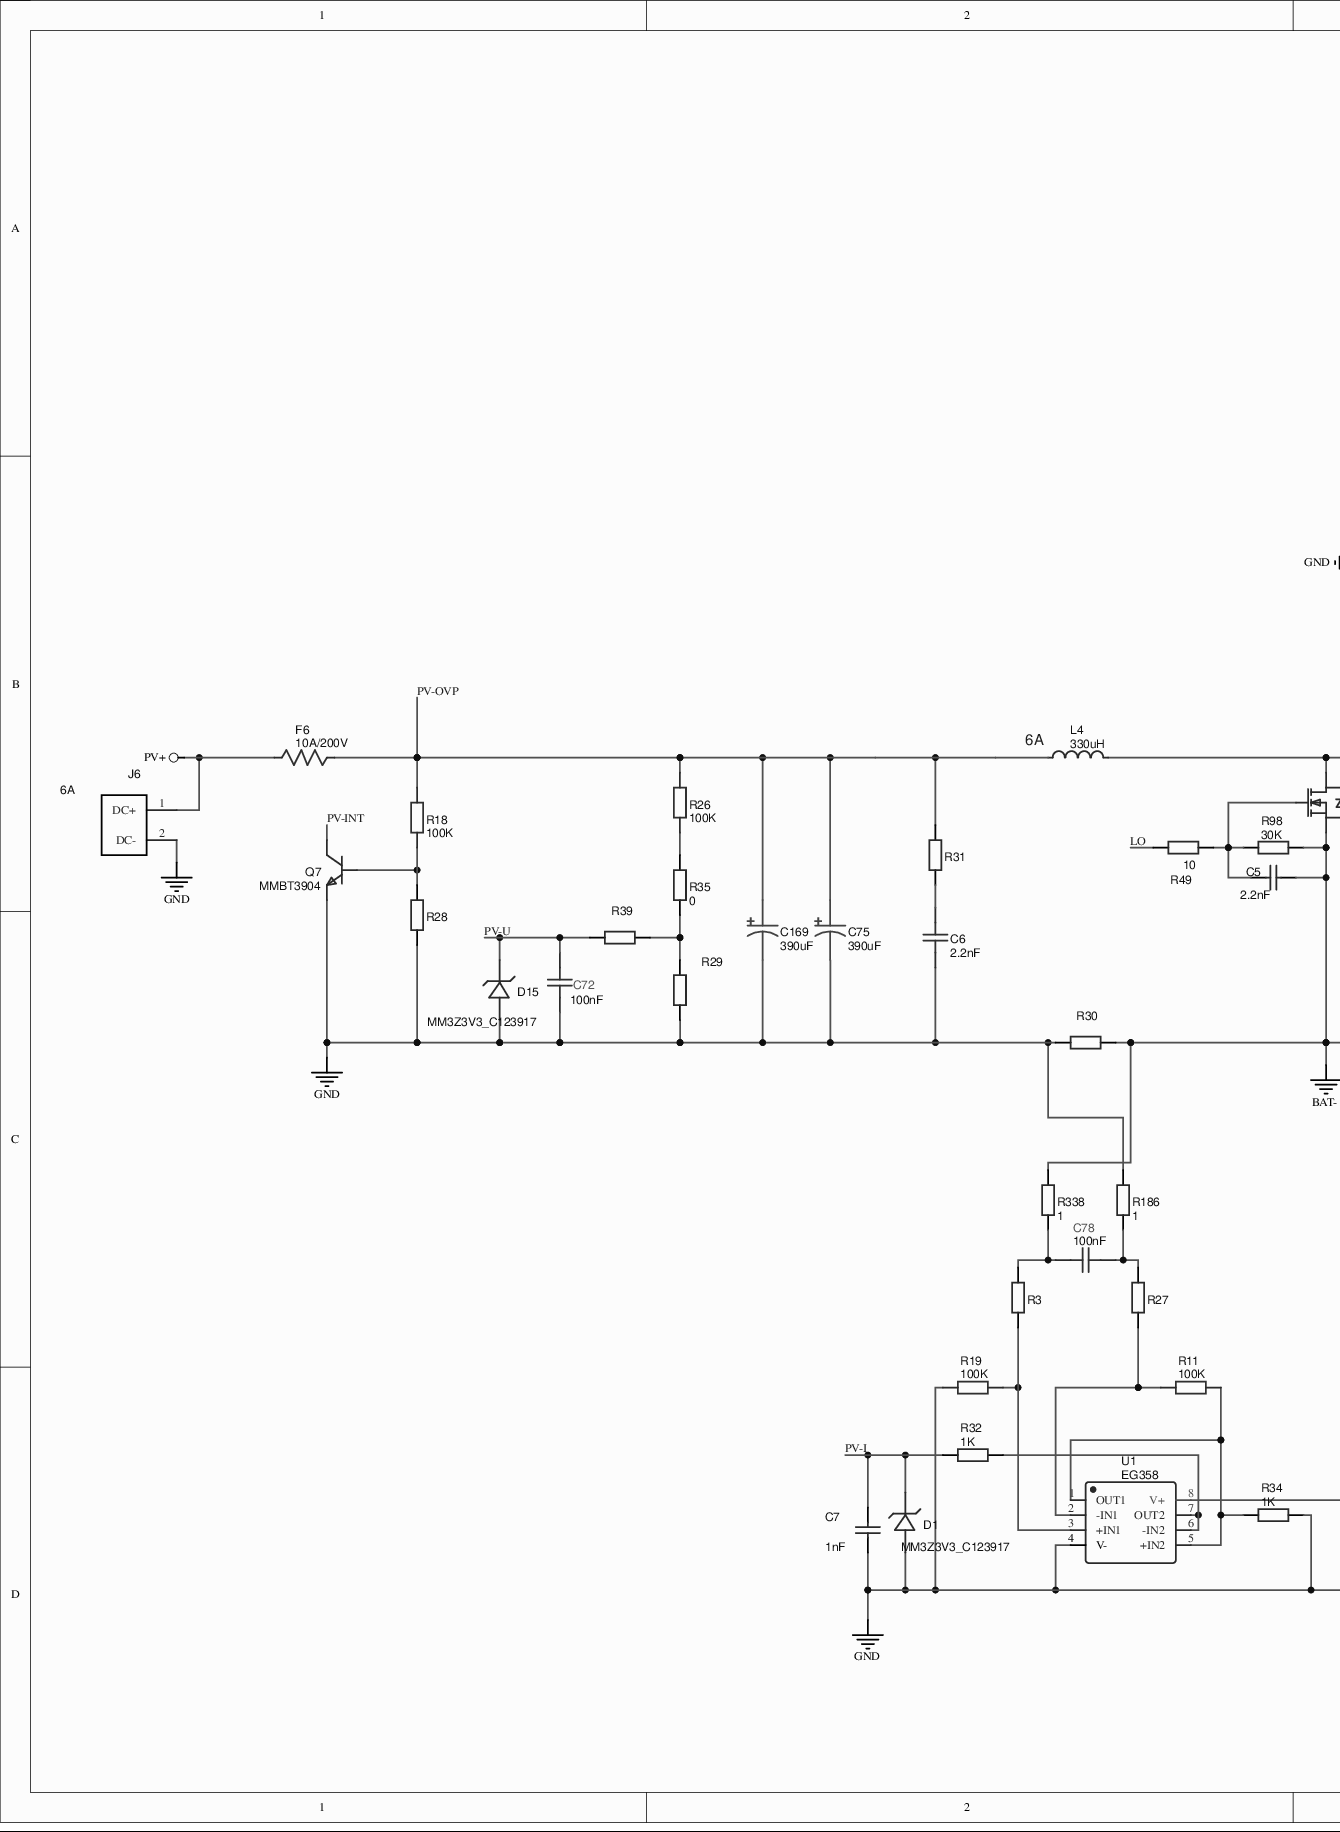
[diagram p0: MISC84449-3.SchDoc, left]
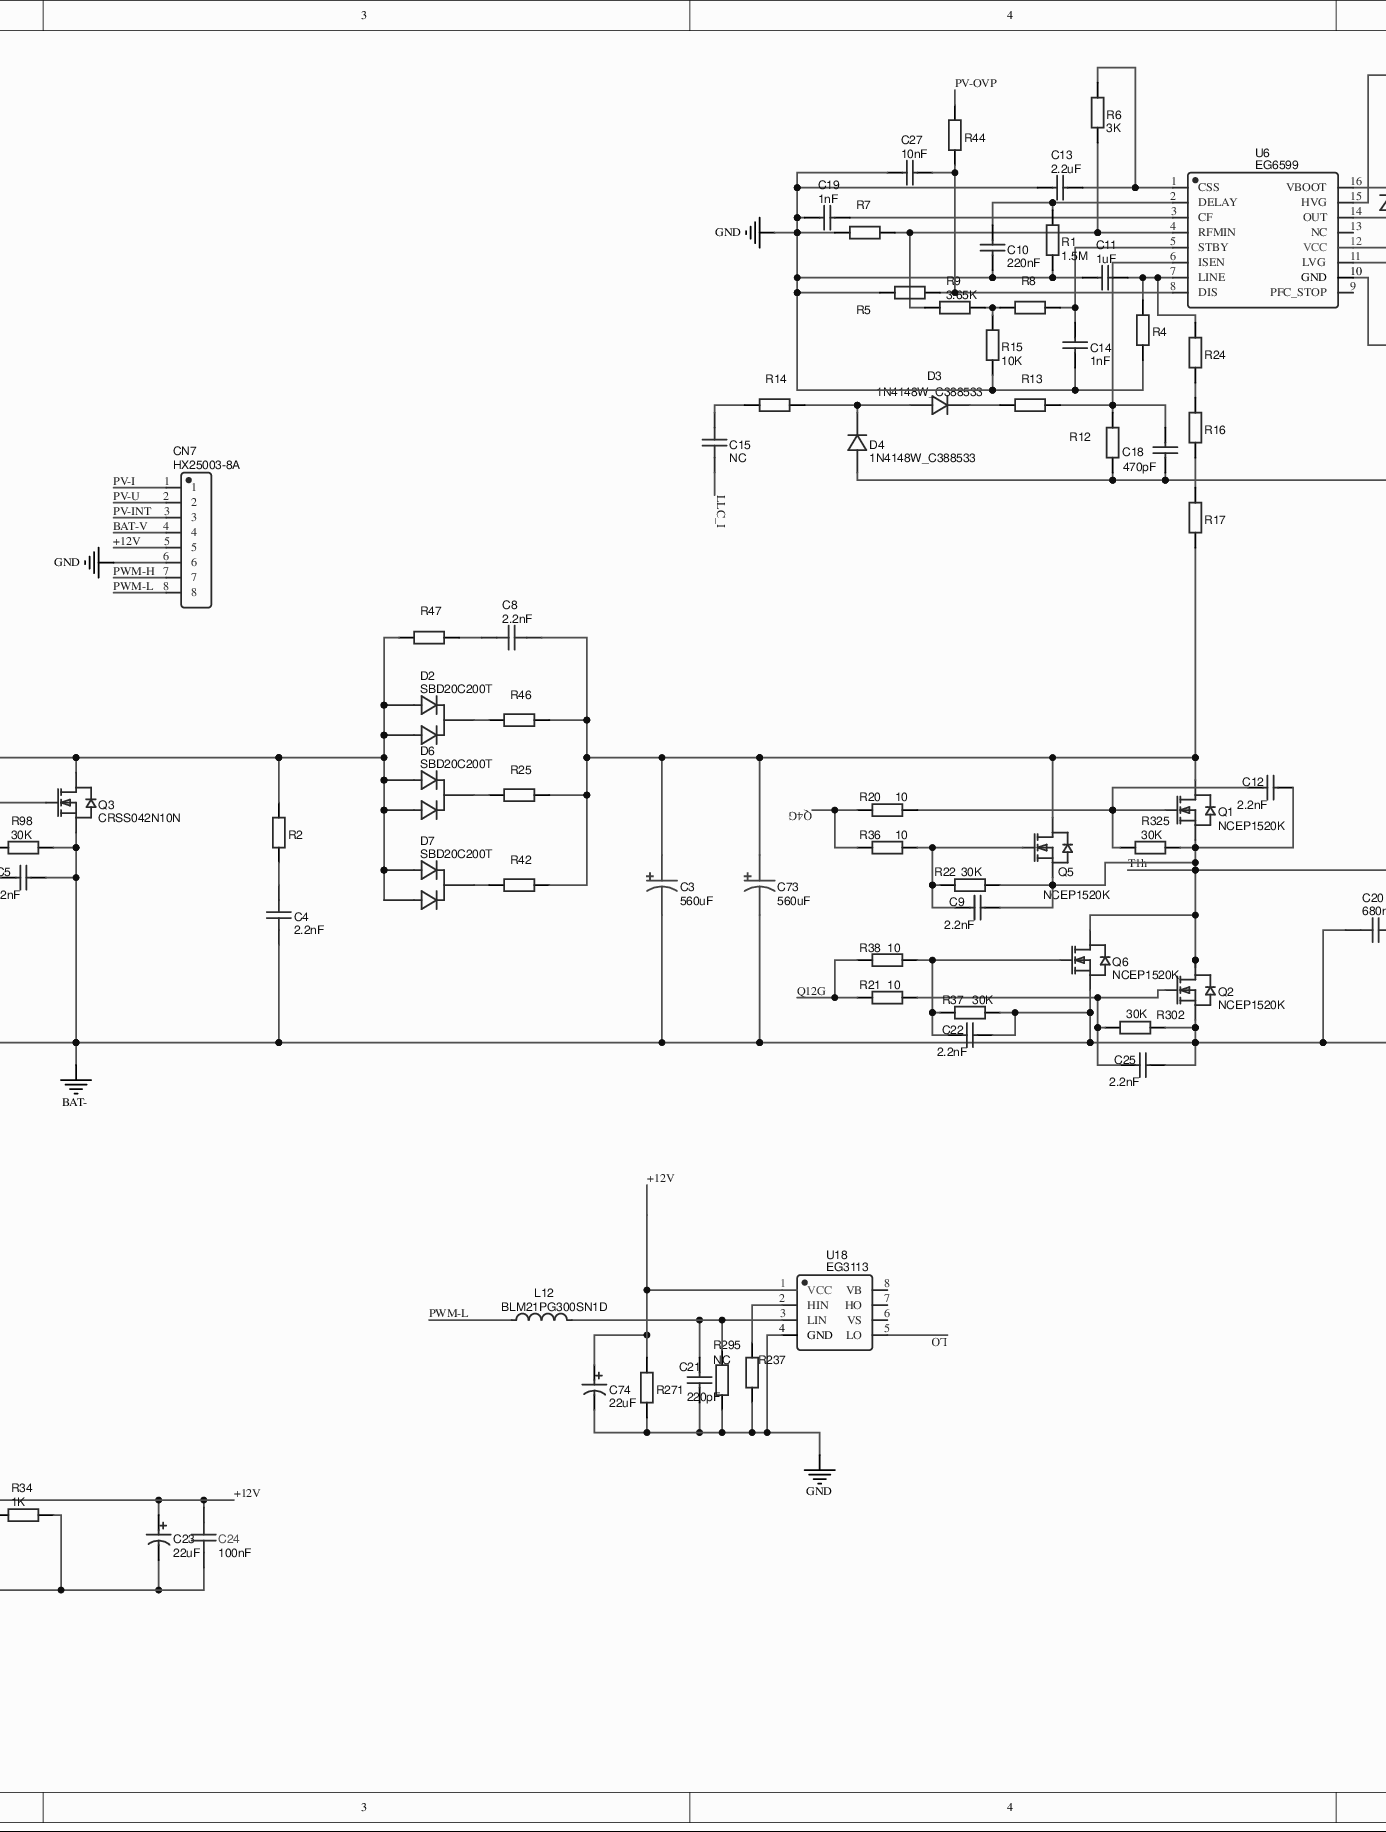
[diagram p1: MISC84449-3.SchDoc, middle]
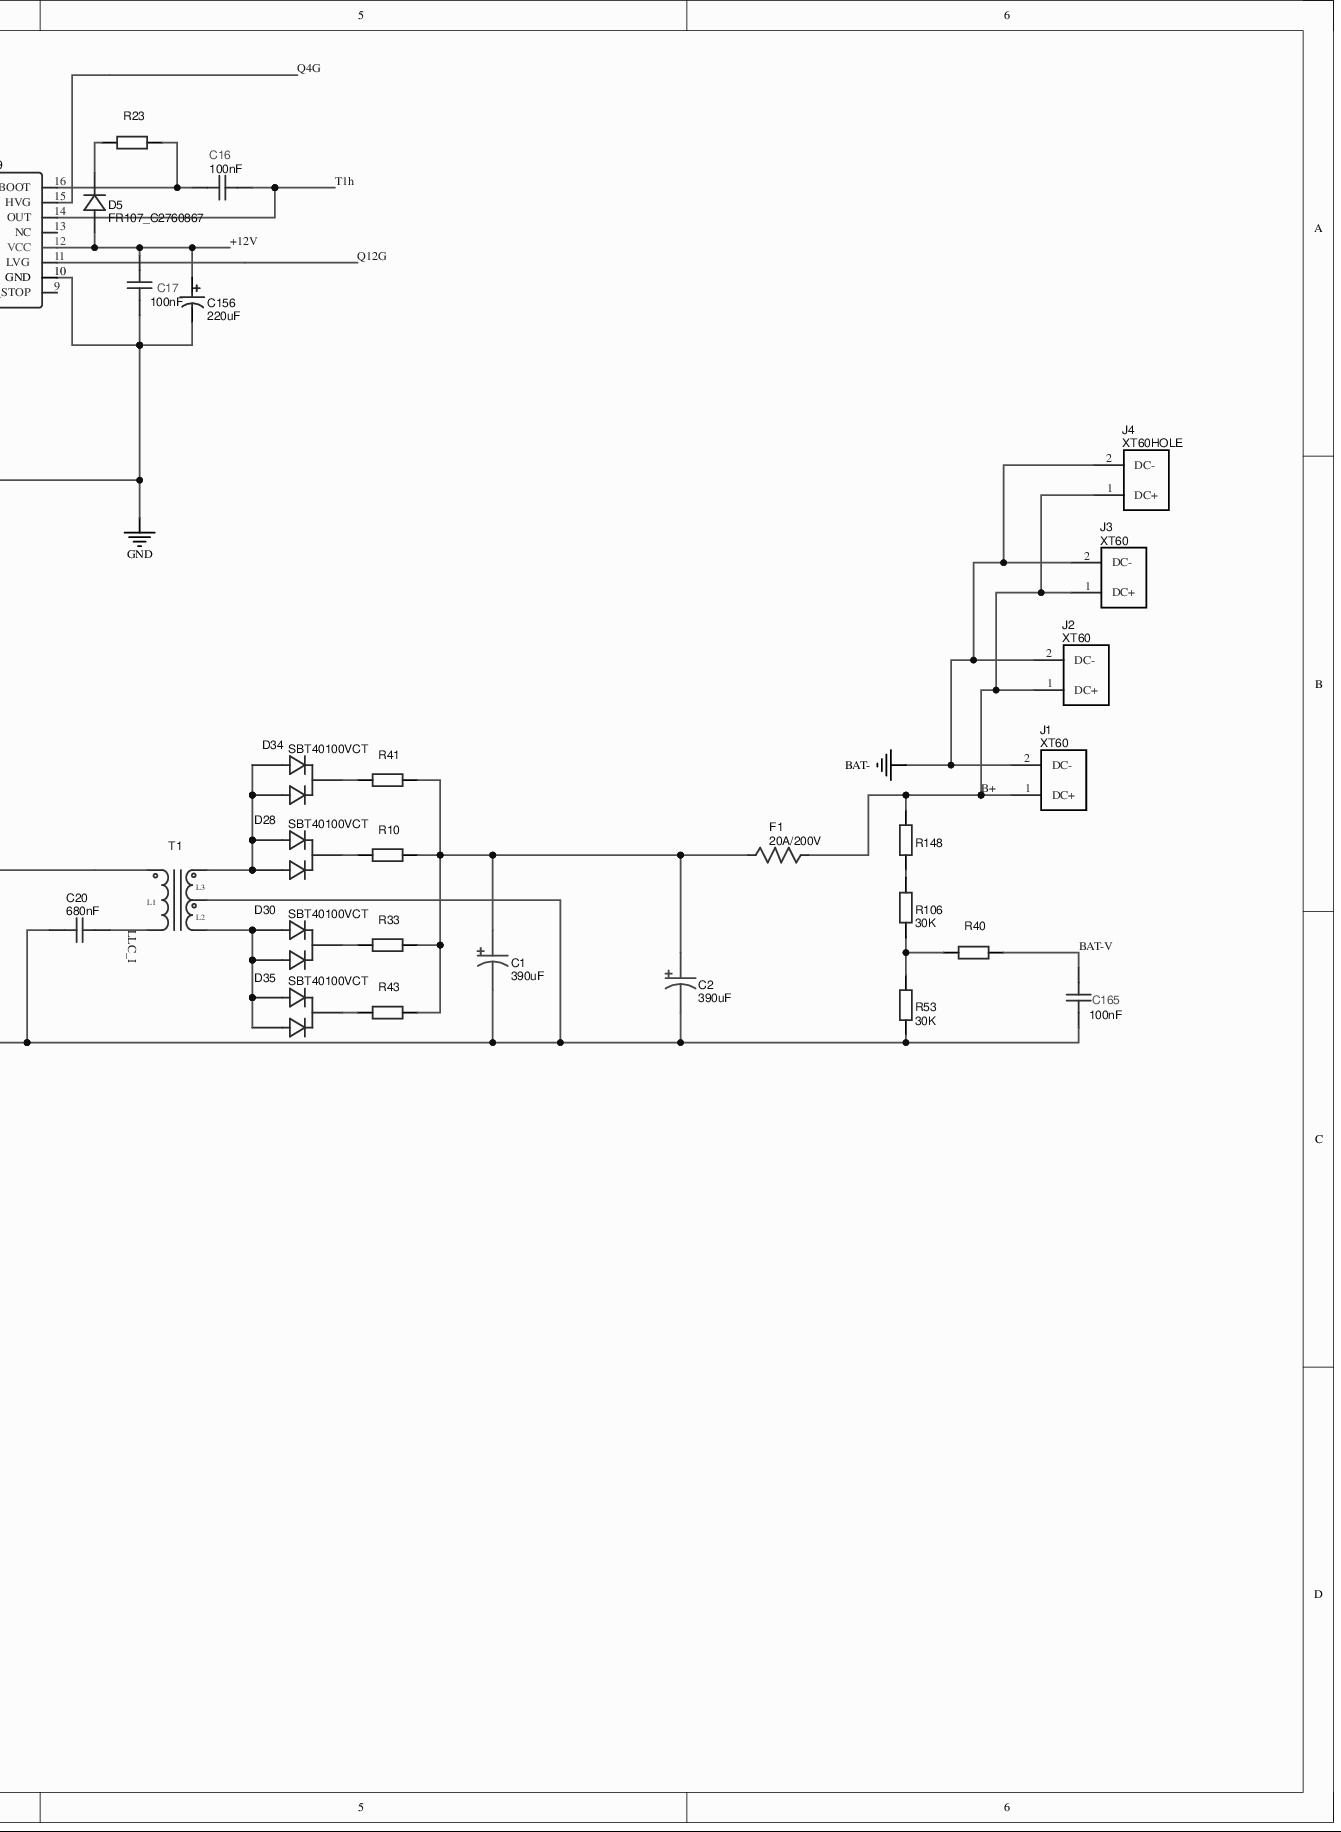
[diagram p2: MISC84449-3.SchDoc, right]
# Altium project MISC84449-4.PrjPcb
1 sheet, 124 parts. Net scope: global (net labels, ports and power ports of the same name join across sheets).
Board file: MISC84449.PcbDoc

## Sheet MISC84449-3.SchDoc
size 655 x 308 mm

### Parts
C1  390uF  [CAP-TH_BD8.0-P3.50-D0.6-FD]
C2  390uF  [CAP-TH_BD8.0-P3.50-D0.6-FD]
C3  560uF  [CAP-TH_BD12.5-P5.00-D0.6-FD]
C4  2.2nF  [C1206]
C5  2.2nF  [C0603]
C6  2.2nF  [C1206]
C7  1nF  [C0603]
C8  2.2nF  [C1206]
C9  2.2nF  [C0603]
C10  220nF  [C0603]
C11  1uF  [C0603]
C12  2.2nF  [C0603]
C13  2.2uF  [C0603]
C14  1nF  [C0603]
C15  NC  [C1206]
C16  100nF  [C0603]
C17  100nF  [C0603]
C18  470pF  [C0603]
C19  1nF  [C0603]
C20  680nF  [CAP-TH_L17.5-W8.5-P15.00-D0.8]
C21  220pF  [C0603]
C22  2.2nF  [C0603]
C23  22uF  [CAP-TH_BD5.0-P2.00-D0.8-FD]
C24  100nF  [C0603]
C25  2.2nF  [C0603]
C27  10nF  [C1206]
C72  100nF  [C0603]
C73  560uF  [CAP-TH_BD12.5-P5.00-D0.6-FD]
C74  22uF  [CAP-TH_BD5.0-P2.00-D0.8-FD]
C75  390uF  [CAP-TH_BD10.0-P5.00-D1.0-FD]
C78  100nF  [C0603]
C156  220uF  [CAP-TH_BD6.3-P2.50-D1.0-FD]
C165  100nF  [C0603]
C169  390uF  [CAP-TH_BD10.0-P5.00-D1.0-FD]
CN7  HX25003-8A  [CONN-TH_8P-P2.50_HX25003-8A]
D1  MM3Z3V3_C123917  [SOD-323_L1.8-W1.3-LS2.5-RD]
D2  SBD20C200T  [TO-220-3_L10.0-W4.5-P2.54-L]
D3  1N4148W_C388533  [SOD-123_L2.8-W1.8-LS3.7-RD]
D4  1N4148W_C388533  [SOD-123_L2.8-W1.8-LS3.7-RD]
D5  FR107_C2760867  [SOD-123FL_L2.7-W1.8-LS3.8-RD]
D6  SBD20C200T  [TO-220-3_L10.0-W4.5-P2.54-L]
D7  SBD20C200T  [TO-220-3_L10.0-W4.5-P2.54-L]
D15  MM3Z3V3_C123917  [SOD-323_L1.8-W1.3-LS2.5-RD]
D28  SBT40100VCT  [TO-220-3_L10.0-W4.5-P2.54-L]
D30  SBT40100VCT  [TO-220-3_L10.0-W4.5-P2.54-L]
D34  SBT40100VCT  [TO-220-3_L10.0-W4.5-P2.54-L]
D35  SBT40100VCT  [TO-220-3_L10.0-W4.5-P2.54-L]
F1  20A/200V  [FUSE-SMD_L6.1-W2.5]
F6  10A/200V  [FUSE-SMD_L6.1-W2.5]
J1  XT60  [CONN-TH_XT60UPB-F]
J2  XT60  [CONN-TH_XT60UPB-F]
J3  XT60  [CONN-TH_XT60UPB-F]
J4  XT60HOLE  [XT90N]
J6  6A  [CONN-TH_XT60UPB-F]
L4  330uH  [200W-TMS330060A]
L12  BLM21PG300SN1D  [L0805]
Q1  NCEP1520K  [TO-252-2_L6.6-W6.1-P4.57-LS9.9-BR-CW]
Q2  NCEP1520K  [TO-252-2_L6.6-W6.1-P4.57-LS9.9-BR-CW]
Q3  CRSS042N10N  [TO-263-3_L10.2-W10.7-P5.08-LS16.2-TL]
Q5  NCEP1520K  [TO-252-2_L6.6-W6.1-P4.57-LS9.9-BR-CW]
Q6  NCEP1520K  [TO-252-2_L6.6-W6.1-P4.57-LS9.9-BR-CW]
Q7  MMBT3904  [SOT-23-3_L2.9-W1.3-P1.90-LS2.4-BR]
R1  1.5M  [R0603]
R2  (no value)  [R1206]
R3  (no value)  [R0603]
R4  (no value)  [R0603]
R5  (no value)  [R0805]
R6  3K  [R0603]
R7  (no value)  [R0603]
R8  (no value)  [R0603]
R9  3.65K  [R0603]
R10  (no value)  [R2512]
R11  100K  [R0805]
R12  (no value)  [R0603]
R13  (no value)  [R0603]
R14  (no value)  [R0603]
R15  10K  [R1206]
R16  (no value)  [R0603]
R17  (no value)  [R1206]
R18  100K  [R0805]
R19  100K  [R0805]
R20  10  [R1206]
R21  10  [R1206]
R22  30K  [R0603]
R23  (no value)  [R0805]
R24  (no value)  [R0603]
R25  (no value)  [R2512]
R26  100K  [R0805]
R27  (no value)  [R0603]
R28  (no value)  [R0805]
R29  (no value)  [R0603]
R30  (no value)  [R2512]
R31  (no value)  [R1206]
R32  1K  [R0603]
R33  (no value)  [R2512]
R34  1K  [R0603]
R35  0  [R0805]
R36  10  [R1206]
R37  30K  [R0603]
R38  10  [R1206]
R39  (no value)  [R0805]
R40  (no value)  [R0805]
R41  (no value)  [R2512]
R42  (no value)  [R2512]
R43  (no value)  [R2512]
R44  (no value)  [R0805]
R46  (no value)  [R2512]
R47  (no value)  [R1206]
R49  10  [R0603]
R53  30K  [R0603]
R98  30K  [R0603]
R106  30K  [R0603]
R148  (no value)  [R0603]
R186  1  [R0603]
R237  (no value)  [R0603]
R271  (no value)  [R0603]
R295  NC  [R0603]
R302  30K  [R0603]
R325  30K  [R0603]
R338  1  [R0603]
T1  (no value)  [PQ3230 3:2:2-N]
U1  EG358  [SOIC-8_L5.0-W4.0-P1.27-LS6.0-BL]
U6  EG6599  [SO-16_L10.0-W4.0-P1.27-LS6.2-BL]
U18  EG3113  [SOP-8_L4.9-W3.9-P1.27-LS6.0-BL]

### Nets
BAT-: C1.2 C2.2 C3.2 C4.2 C5.2 C20.2 C22.2 C25.2 C73.2 C165.1 J1.2(DC-) J2.2(DC-) J3.2(DC-) J4.2(DC-) Q2.3(S) Q3.3(S) Q6.3(S) R30.2 R37.2 R53.1 R98.1 R302.2 R338.2 T1.9
GND: C6.2 C7.1 C10.1 C11.2 C13.1 C14.1 C17.1 C18.1 C19.2 C21.1 C23.2 C24.2 C27.1 C72.1 C74.2 C75.2 C156.2 C169.2 CN7.6 D1.2(A) D4.2(A) D15.2(A) J6.2(DC-) Q7.2(E) R1.1 R4.1 R5.1 R7.2 R12.1 R15.2 R19.2 R28.1 R29.1 R30.1 R34.2 R186.2 R237.1 R271.1 R295.2 U1.4(V-) U6.10(GND) U18.4(GND)
PV+: F6.1 J6.1(DC+)
+12V: C17.2 C23.1 C24.1 C74.1 C156.1 CN7.5 D5.2(A) R271.2 U1.8(V+) U6.12(VCC) U18.1(VCC)
B+: F1.2 J1.1(DC+) J2.1(DC+) J3.1(DC+) J4.1(DC+) R148.2
BAT-V: C165.2 CN7.4 R40.2
LLC_I: C15.1 C20.1 T1.3
LO: R49.2 U18.5(LO)
PV-I: C7.2 CN7.1 D1.1(K) R32.2
PV-INT: CN7.3 Q7.3(C)
PV-OVP: C75.1 C169.1 F6.2 L4.1 R18.2 R26.2 R31.1 R44.2
PV-U: C72.2 CN7.2 D15.1(K) R39.1
PWM-H: CN7.7
PWM-L: CN7.8 L12.1
Q4G: R20.1 R36.1 U6.15(HVG)
Q12G: R21.1 R38.1 U6.11(LVG)
T1h: C9.2 C12.2 C16.1 Q1.3(S) Q2.2(D) Q5.3(S) Q6.2(D) R22.2 R325.2 T1.4 U6.14(OUT)
NetC1_1: C1.1 C2.1 F1.1 R10.2 R33.2 R41.2 R43.2
NetC3_1: C3.1 C8.2 C73.1 Q1.2(D) Q5.2(D) R17.1 R25.2 R42.2 R46.2
NetC4_1: C4.1 R2.2
NetC5_1: C5.1 Q3.1(G) R49.1 R98.2
NetC6_1: C6.1 R31.2
NetC8_1: C8.1 R47.2
NetC9_1: C9.1 Q5.1(G) R22.1 R36.2
NetC10_2: C10.2 R1.2 U6.2(DELAY)
NetC11_1: C11.1 R4.2 R24.2 U6.7(LINE)
NetC12_1: C12.1 Q1.1(G) R20.2 R325.1
NetC13_2: C13.2 R6.2 U6.1(CSS)
NetC14_2: C14.2 R8.2 U6.5(STBY)
NetC15_2: C15.2 R14.1
NetC16_2: C16.2 R23.1 U6.16(VBOOT)
NetC18_2: C18.2 R12.2 R13.2 U6.6(ISEN)
NetC19_1: C19.1 U6.3(CF)
NetC21_2: C21.2 L12.2 R295.1 U18.3(LIN)
NetC22_1: C22.1 Q6.1(G) R37.1 R38.2
NetC25_1: C25.1 Q2.1(G) R21.2 R302.1
NetC27_2: C27.2 R5.2 R44.1 U6.8(DIS)
NetC78_1: C78.1 R27.2 R186.1
NetC78_2: C78.2 R3.2 R338.1
NetD2_1: D2.1 D2.3 D6.1 D6.3 D7.1 D7.3 L4.2 Q3.2(D) R2.1 R47.1
NetD2_2: D2.2 R46.1
NetD3_1: D3.1(C) R13.1
NetD3_2: D3.2(A) D4.1(C) R14.2
NetD5_1: D5.1(K) R23.2
NetD6_2: D6.2 R25.1
NetD7_2: D7.2 R42.1
NetD28_1: D28.1 D28.3 D34.1 D34.3 T1.8
NetD28_2: D28.2 R10.1
NetD30_1: D30.1 D30.3 D35.1 D35.3 T1.10
NetD30_2: D30.2 R33.1
NetD34_2: D34.2 R41.1
NetD35_2: D35.2 R43.1
NetQ7_1: Q7.1(B) R18.1 R28.2
NetR3_1: R3.1 R19.1 U1.3(+IN1)
NetR6_1: R6.1 R7.1 R9.1 U6.4(RFMIN)
NetR8_1: R8.1 R9.2 R15.1
NetR11_1: R11.1 R34.1 U1.1(OUT1) U1.5(+IN2)
NetR11_2: R11.2 R27.1 U1.2(-IN1)
NetR16_1: R16.1 R17.2
NetR16_2: R16.2 R24.1
NetR26_1: R26.1 R35.2
NetR29_2: R29.2 R35.1 R39.2
NetR32_1: R32.1 U1.6(-IN2) U1.7(OUT2)
NetR40_1: R40.1 R53.2 R106.1
NetR106_2: R106.2 R148.1
NetR237_2: R237.2 U18.2(HIN)

Not connected (* = marked no-connect by the designer): U6 9(PFC_STOP) 13(NC); U18 6(VS) 7(HO) 8(VB)

### Notes on the sheet
- (near L4) 6A

### Library data of the parts
C1 C2 = 390uF: BOM_Manufacturer: Ymin; BOM_Manufacturer Part: LKMD1601V391MF; nameAlias: Capacitance; Contributor: LCSC; BOM_Supplier: LCSC; BOM_Supplier Part: C442877; BOM_JLCPCB Part Class: Extended Part; spicePre: C; spiceSymbolName: LKMD1601V391MF
C3 C73 = 560uF: BOM_Manufacturer: PANASONIC; BOM_Manufacturer Part: EEUFS1J561; nameAlias: Capacitance; Contributor: LCSC; BOM_Supplier: LCSC; BOM_Supplier Part: C178687; BOM_JLCPCB Part Class: Extended Part; spicePre: C; spiceSymbolName: EEUFS1J561
C4 C6 C8 = 2.2nF: BOM_Manufacturer: Johanson Dielectrics; BOM_Manufacturer Part: 202R18W222KV4E; nameAlias: Capacitance; Contributor: LCSC; BOM_Supplier: LCSC; BOM_Supplier Part: C173213; BOM_JLCPCB Part Class: Extended Part; spicePre: C; spiceSymbolName: 202R18W222KV4E
C5 C9 C12 C22 C25 = 2.2nF: BOM_Manufacturer: YAGEO; BOM_Manufacturer Part: CC0603KRX7R9BB222; nameAlias: Capacitance; BOM_Supplier: LCSC; BOM_Supplier Part: C107082; BOM_JLCPCB Part Class: Extended Part; spicePre: C; spiceSymbolName: CC0603KRX7R9BB222
C7 C14 = 1nF: BOM_Manufacturer Part: CL10B102KB8NNNC; BOM_Manufacturer: SAMSUNG; nameAlias: Capacitance; BOM_Supplier: LCSC; BOM_Supplier Part: C1588; BOM_JLCPCB Part Class: Basic Part; spicePre: C; spiceSymbolName: CL10B102KB8NNNC
C10 = 220nF: BOM_Manufacturer Part: CL10B224KA8NNNC; BOM_Manufacturer: SAMSUNG; nameAlias: Capacitance; BOM_Supplier: LCSC; BOM_Supplier Part: C21120; BOM_JLCPCB Part Class: Basic Part; spicePre: C; spiceSymbolName: CL10B224KA8NNNC
C11 = 1uF: BOM_Manufacturer Part: CL10A105KB8NNNC; BOM_Manufacturer: SAMSUNG; nameAlias: Capacitance; BOM_Supplier: LCSC; BOM_Supplier Part: C15849; BOM_JLCPCB Part Class: Basic Part; spicePre: C; spiceSymbolName: CL10A105KB8NNNC
C13 = 2.2uF: BOM_Manufacturer Part: CL10A225KO8NNNC; BOM_Manufacturer: SAMSUNG; nameAlias: Capacitance; BOM_Supplier: LCSC; BOM_Supplier Part: C23630; BOM_JLCPCB Part Class: Basic Part; spicePre: C; spiceSymbolName: CL10A225KO8NNNC
C15 = NC: BOM_Manufacturer: Guangdong Fenghua Advanced Tech; BOM_Manufacturer Part: 1206CG220J102NT; nameAlias: Capacitance; Contributor: LCSC; BOM_Supplier: LCSC; BOM_Supplier Part: C313096; BOM_JLCPCB Part Class: Extended Part; spicePre: C; spiceSymbolName: 1206CG220J102NT
C16 C17 C24 C72 C78 C165 = 100nF: BOM_Manufacturer: SAMSUNG; BOM_Manufacturer Part: CL10B104KC8NNNC; nameAlias: Capacitance; BOM_Supplier: LCSC; BOM_Supplier Part: C15725; BOM_JLCPCB Part Class: Extended Part; spicePre: C; spiceSymbolName: CL10B104KC8NNNC
C18 = 470pF: BOM_Manufacturer: FH; BOM_Manufacturer Part: 0603B471K500NT; nameAlias: Capacitance; BOM_Supplier: LCSC; BOM_Supplier Part: C1620; BOM_JLCPCB Part Class: Basic Part; spicePre: C; spiceSymbolName: 0603B471K500NT
C19 = 1nF: BOM_Manufacturer: SAMSUNG; BOM_Manufacturer Part: CL10B102KB8NNNC; nameAlias: Capacitance; Contributor: LCSC; BOM_Supplier: LCSC; BOM_Supplier Part: C1588; BOM_JLCPCB Part Class: Extended Part; spicePre: C; spiceSymbolName: CL10B102KC8NNNC
C20 = 680nF: BOM_Manufacturer: KYET; BOM_Manufacturer Part: KP684J2J1502; nameAlias: Capacitance; Contributor: LCSC; BOM_Supplier: LCSC; BOM_Supplier Part: C390149; BOM_JLCPCB Part Class: Extended Part; spicePre: C; spiceSymbolName: KP684J2J1502
C21 = 220pF: BOM_Manufacturer: YAGEO; BOM_Manufacturer Part: CC0603KRX7R9BB221; nameAlias: Capacitance; BOM_Supplier: LCSC; BOM_Supplier Part: C107081; BOM_JLCPCB Part Class: Extended Part; spicePre: C; spiceSymbolName: CC0603KRX7R9BB221
C23 C74 = 22uF: BOM_Manufacturer: ValuePro; BOM_Manufacturer Part: 22uF 50V 5*11; nameAlias: Capacitance; BOM_Supplier: LCSC; BOM_Supplier Part: C43346; BOM_JLCPCB Part Class: Extended Part; spicePre: C; spiceSymbolName: 22uF 50V 5*11
C27 = 10nF: BOM_Manufacturer: FH; BOM_Manufacturer Part: 1206B103K102NT; nameAlias: Capacitance; BOM_Supplier: LCSC; BOM_Supplier Part: C9194; BOM_JLCPCB Part Class: Extended Part; spicePre: C; spiceSymbolName: 1206B103K102NT
C75 C169 = 390uF: BOM_Manufacturer: Ymin; BOM_Manufacturer Part: LKME2001J391MF; nameAlias: Capacitance; Contributor: LCSC; BOM_Supplier: LCSC; BOM_Supplier Part: C442948; BOM_JLCPCB Part Class: Extended Part; spicePre: C; spiceSymbolName: LKME2001J391MF
C156 = 220uF: BOM_Manufacturer: ValuePro; BOM_Manufacturer Part: 220uF 16V 6.3*11; nameAlias: Capacitance; BOM_Supplier: LCSC; BOM_Supplier Part: C43349; BOM_JLCPCB Part Class: Extended Part; spicePre: C; spiceSymbolName: 220uF 16V 6.3*11
CN7 = HX25003-8A: BOM_Manufacturer: HX(Zhejiang Yueqing Hongxing Elec); Contributor: LCSC; BOM_Supplier: LCSC; BOM_Supplier Part: C442305; BOM_Manufacturer Part: HX25003-8A; BOM_JLCPCB Part Class: Extended Part; spicePre: C; spiceSymbolName: HX25003-8A
D1 D15 = MM3Z3V3_C123917: BOM_Manufacturer: Shandong Jingdao Microelectronics; Contributor: LCSC; BOM_Supplier: LCSC; BOM_Supplier Part: C123917; BOM_Manufacturer Part: MM3Z3V3; BOM_JLCPCB Part Class: Extended Part; spicePre: D; spiceSymbolName: MM3Z3V3_C123917
D2 D6 D7 = SBD20C200T: BOM_Manufacturer: PANJIT; BOM_Manufacturer Part: SBT40100VCT; Contributor: LCSC; BOM_Supplier Part: C142331; BOM_Supplier: LCSC; BOM_JLCPCB Part Class: Extended Part; spicePre: D; spiceSymbolName: SBT40100VCT
D3 D4 = 1N4148W_C388533: BOM_Manufacturer: Yangzhou Yangjie Elec Tech; Contributor: LCSC; BOM_Supplier: LCSC; BOM_Supplier Part: C388533; BOM_Manufacturer Part: 1N4148W; BOM_JLCPCB Part Class: Extended Part; spicePre: D; spiceSymbolName: 1N4148W_C388533
D5 = FR107_C2760867: BOM_Manufacturer Part: FR107; Contributor: LCSC; BOM_Supplier: LCSC; BOM_Supplier Part: C2760867; BOM_JLCPCB Part Class: Extended Part; spicePre: D; spiceSymbolName: FR107_C2760867
D28 D30 D34 D35 = SBT40100VCT: BOM_Manufacturer: PANJIT; Contributor: LCSC; BOM_Supplier Part: C142331; BOM_Supplier: LCSC; BOM_Manufacturer Part: SBT40100VCT; BOM_JLCPCB Part Class: Extended Part; spicePre: D; spiceSymbolName: SBT40100VCT
F1 = 20A/200V: Contributor: LCEDA_Lib; spicePre: R; spiceSymbolName: R_1206_US
F6 = 10A/200V: Contributor: LCEDA_Lib; spicePre: R; spiceSymbolName: R_1206_US
J1-J3 = XT60: BOM_Manufacturer: ReliaPro; BOM_Manufacturer Part: TJC1-2A; BOM_Supplier: LCSC; BOM_Supplier Part: C29632; spicePre: J; spiceSymbolName: TJC1-2A
J4 = XT60HOLE: BOM_Manufacturer: ReliaPro; BOM_Manufacturer Part: TJC1-2A; BOM_Supplier: LCSC; BOM_Supplier Part: C29632; spicePre: J; spiceSymbolName: TJC1-2A
J6 = 6A: BOM_Manufacturer: ReliaPro; BOM_Manufacturer Part: TJC1-2A; BOM_Supplier: LCSC; BOM_Supplier Part: C29632; spicePre: J; spiceSymbolName: TJC1-2A
L4 = 330uH: nameAlias: Value(H); Contributor: LCEDA_Lib; spicePre: L; spiceSymbolName: L0402_US
L12 = BLM21PG300SN1D: BOM_Manufacturer: MuRata; nameAlias: Value(H); BOM_Supplier: LCSC; BOM_Manufacturer Part: BLM21PG300SN1D; BOM_Supplier Part: C16903; BOM_JLCPCB Part Class: Extended Part; spicePre: L; spiceSymbolName: BLM21PG300SN1D
Q1 Q2 Q5 Q6 = NCEP1520K: BOM_Manufacturer: Wuxi NCE Power Semiconductor; Contributor: LCSC; BOM_Supplier: LCSC; BOM_Supplier Part: C341717; BOM_Manufacturer Part: NCEP1520K; BOM_JLCPCB Part Class: Extended Part; spicePre: Q; spiceSymbolName: NCEP1520K
Q3 = CRSS042N10N: BOM_Manufacturer: CRMICRO; Contributor: LCSC; BOM_Supplier: LCSC; BOM_Supplier Part: C410926; BOM_Manufacturer Part: CRSS042N10N; BOM_JLCPCB Part Class: Extended Part; spicePre: Q; spiceSymbolName: CRSS042N10N
Q7 = MMBT3904: Contributor: LCSC; BOM_Supplier: LCSC; BOM_Supplier Part: C2688228; BOM_Manufacturer Part: MMBT3904; BOM_JLCPCB Part Class: Extended Part; spicePre: Q; spiceSymbolName: MMBT3904
R1 = 1.5M: BOM_Manufacturer: YAGEO; BOM_Manufacturer Part: RC0603FR-071M5L; nameAlias: Resistance (Ohms); BOM_Supplier: LCSC; BOM_Supplier Part: C137773; BOM_JLCPCB Part Class: Extended Part; spicePre: R; spiceSymbolName: RC0603FR-071M5L
R2 R31 R47 = (no symbol name): BOM_Manufacturer: UniOhm; BOM_Manufacturer Part: 1206W4F100KT5E; nameAlias: Resistance; Resistance (Ohms): 1; BOM_Supplier: LCSC; BOM_Supplier Part: C17928; BOM_JLCPCB Part Class: Basic Part; spicePre: R; spiceSymbolName: 1206W4F100KT5E
R3 R12 R27 = (no symbol name): BOM_Manufacturer: UniOhm; BOM_Manufacturer Part: 0603WAF1501T5E; nameAlias: Resistance; Resistance (Ohms): 1.5K; BOM_Supplier: LCSC; BOM_Supplier Part: C22843; BOM_JLCPCB Part Class: Basic Part; spicePre: R; spiceSymbolName: 0603WAF1501T5E
R4 R14 R16 R24 R271 = (no symbol name): BOM_Manufacturer: UniOhm; BOM_Manufacturer Part: 0603WAF1002T5E; nameAlias: Resistance; Resistance (Ohms): 10K; BOM_Supplier: LCSC; BOM_Supplier Part: C25804; BOM_JLCPCB Part Class: Basic Part; spicePre: R; spiceSymbolName: 0603WAF1002T5E
R5 = (no symbol name): BOM_Manufacturer: UniOhm; BOM_Manufacturer Part: 0805W8F9101T5E; nameAlias: Resistance; Resistance (Ohms): 9.1K; BOM_Supplier: LCSC; BOM_Supplier Part: C17855; BOM_JLCPCB Part Class: Basic Part; spicePre: R; spiceSymbolName: 0805W8F9101T5E
R6 = 3K: BOM_Manufacturer: YAGEO; BOM_Manufacturer Part: RC0603FR-073KL; nameAlias: Resistance (Ohms); BOM_Supplier: LCSC; BOM_Supplier Part: C126358; BOM_JLCPCB Part Class: Extended Part; spicePre: R; spiceSymbolName: RC0603FR-073KL
R7 R29 = (no symbol name): BOM_Manufacturer: UniOhm; BOM_Manufacturer Part: 0603WAF4701T5E; nameAlias: Resistance; Resistance (Ohms): 4.7K; BOM_Supplier: LCSC; BOM_Supplier Part: C23162; BOM_JLCPCB Part Class: Basic Part; spicePre: R; spiceSymbolName: 0603WAF4701T5E
R8 R237 = (no symbol name): BOM_Manufacturer: UniOhm; BOM_Manufacturer Part: 0603WAF0000T5E; nameAlias: Resistance; Resistance (Ohms): 0; BOM_Supplier: LCSC; BOM_Supplier Part: C21189; BOM_JLCPCB Part Class: Basic Part; spicePre: R; spiceSymbolName: 0603WAF0000T5E
R9 = 3.65K: BOM_Manufacturer: YAGEO; BOM_Manufacturer Part: RC0603FR-073K65L; nameAlias: Resistance (Ohms); BOM_Supplier: LCSC; BOM_Supplier Part: C137730; BOM_JLCPCB Part Class: Extended Part; spicePre: R; spiceSymbolName: RC0603FR-073K65L
R10 R25 R33 R41-R43 R46 = (no symbol name): BOM_Manufacturer: RALEC; BOM_Manufacturer Part: RTT25R100FTE; nameAlias: Resistance; Resistance (Ohms): 0.1; BOM_Supplier: LCSC; BOM_Supplier Part: C105145; BOM_JLCPCB Part Class: Extended Part; spicePre: R; spiceSymbolName: RTT25R100FTE
R11 R18 R19 R26 = 100K: BOM_Manufacturer: YAGEO; BOM_Manufacturer Part: RC0805JR-07100KL; nameAlias: Resistance (Ohms); Contributor: LCSC; BOM_Supplier: LCSC; BOM_Supplier Part: C100049; BOM_JLCPCB Part Class: Extended Part; spicePre: R; spiceSymbolName: RC0805JR-07100KL
R13 = (no symbol name): BOM_Manufacturer: UniOhm; BOM_Manufacturer Part: 0603WAF510JT5E; nameAlias: Resistance; Resistance (Ohms): 51; BOM_Supplier: LCSC; BOM_Supplier Part: C23197; BOM_JLCPCB Part Class: Basic Part; spicePre: R; spiceSymbolName: 0603WAF510JT5E
R15 = 10K: BOM_Manufacturer: UniOhm; BOM_Manufacturer Part: 1206W4F1002T5E; nameAlias: Resistance (Ohms); BOM_Supplier: LCSC; BOM_Supplier Part: C17902; BOM_JLCPCB Part Class: Basic Part; spicePre: R; spiceSymbolName: 1206W4F1002T5E
R17 = (no symbol name): BOM_Manufacturer: UniOhm; BOM_Manufacturer Part: 1206W4F3003T5E; nameAlias: Resistance; Resistance (Ohms): 300K; BOM_Supplier: LCSC; BOM_Supplier Part: C17884; BOM_JLCPCB Part Class: Extended Part; spicePre: R; spiceSymbolName: 1206W4F3003T5E
R20 R21 R36 R38 = 10: BOM_Manufacturer: LIZ; BOM_Manufacturer Part: CR1206J40100G; nameAlias: Resistance (Ohms); BOM_Supplier: LCSC; BOM_Supplier Part: C102266; BOM_JLCPCB Part Class: Extended Part; spicePre: R; spiceSymbolName: CR1206J40100G
R22 R37 R53 R98 R106 R302 R325 = 30K: BOM_Manufacturer: UniOhm; BOM_Manufacturer Part: 0805W8F3002T5E; nameAlias: Resistance (Ohms); BOM_Supplier: LCSC; BOM_Supplier Part: C17621; BOM_JLCPCB Part Class: Basic Part; spicePre: R; spiceSymbolName: 0805W8F3002T5E
R23 = (no symbol name): BOM_Manufacturer: UniOhm; BOM_Manufacturer Part: 0805W8F220KT5E; nameAlias: Resistance; Resistance (Ohms): 2.2; BOM_Supplier: LCSC; BOM_Supplier Part: C17521; BOM_JLCPCB Part Class: Basic Part; spicePre: R; spiceSymbolName: 0805W8F220KT5E
R28 = (no symbol name): BOM_Manufacturer: FH; BOM_Manufacturer Part: RS-05K1002FT; nameAlias: Resistance; Resistance (Ohms): 10K; BOM_Supplier: LCSC; BOM_Supplier Part: C115309; BOM_JLCPCB Part Class: Extended Part; spicePre: R; spiceSymbolName: RS-05K1002FT
R30 = (no symbol name): BOM_Manufacturer: PSA; BOM_Manufacturer Part: FMF25FPHR005-LHL; nameAlias: Resistance; Resistance (Ohms): 0.005; BOM_Supplier: LCSC; BOM_Supplier Part: C105361; BOM_JLCPCB Part Class: Extended Part; spicePre: R; spiceSymbolName: FMF25FPHR005-LHL
R32 R34 = 1K: BOM_Manufacturer: FH; BOM_Manufacturer Part: RS-03K102JT; nameAlias: Resistance (Ohms); BOM_Supplier: LCSC; BOM_Supplier Part: C73797; spicePre: R; spiceSymbolName: RS-03K102JT
R35 = 0: BOM_Manufacturer: YAGEO; BOM_Manufacturer Part: RC0805FR-070RL; nameAlias: Resistance (Ohms); BOM_Supplier: LCSC; BOM_Supplier Part: C100045; BOM_JLCPCB Part Class: Extended Part; spicePre: R; spiceSymbolName: RC0805FR-070RL
R39 R40 = (no symbol name): BOM_Manufacturer: UniOhm; BOM_Manufacturer Part: 0805W8F1001T5E; nameAlias: Resistance; Resistance (Ohms): 1K; BOM_Supplier: LCSC; BOM_Supplier Part: C17513; BOM_JLCPCB Part Class: Basic Part; spicePre: R; spiceSymbolName: 0805W8F1001T5E
R44 = (no symbol name): BOM_Manufacturer: UniOhm; BOM_Manufacturer Part: 0805W8F2323T5E; nameAlias: Resistance; Resistance (Ohms): 232K; BOM_Supplier: LCSC; BOM_Supplier Part: C17566; BOM_JLCPCB Part Class: Extended Part; spicePre: R; spiceSymbolName: 0805W8F2323T5E
R49 = 10: BOM_Manufacturer: UniOhm; BOM_Manufacturer Part: 0805W8F100JT5E; nameAlias: Resistance (Ohms); BOM_Supplier: LCSC; BOM_Supplier Part: C17415; BOM_JLCPCB Part Class: Basic Part; spicePre: R; spiceSymbolName: 0805W8F100JT5E
R148 = (no symbol name): BOM_Manufacturer: UniOhm; BOM_Manufacturer Part: 0603WAF2703T5E; nameAlias: Resistance; Resistance (Ohms): 270K; BOM_Supplier: LCSC; BOM_Supplier Part: C22965; BOM_JLCPCB Part Class: Basic Part; spicePre: R; spiceSymbolName: 0603WAF2703T5E
R186 R338 = 1: BOM_Manufacturer: YAGEO; BOM_Manufacturer Part: RC0805FR-071RL; nameAlias: Resistance (Ohms); BOM_Supplier: LCSC; BOM_Supplier Part: C131397; BOM_JLCPCB Part Class: Extended Part; spicePre: R; spiceSymbolName: RC0805FR-071RL
R295 = NC: BOM_Manufacturer: FH; BOM_Manufacturer Part: RS-03K102JT; nameAlias: Resistance (Ohms); BOM_Supplier: LCSC; BOM_Supplier Part: C73797; spicePre: R; spiceSymbolName: RS-03K102JT
T1 = (no symbol name): Contributor: z123tt; spicePre: U
U1 = EG358: BOM_Manufacturer: EG; BOM_Supplier: LCSC; BOM_Manufacturer Part: EG358; BOM_Supplier Part: C111033; BOM_JLCPCB Part Class: Extended Part; spicePre: U; spiceSymbolName: EG358
U6 = EG6599: BOM_Manufacturer: EG Micro; Contributor: LCSC; BOM_Supplier: LCSC; BOM_Supplier Part: C481167; BOM_Manufacturer Part: EG6599; BOM_JLCPCB Part Class: Extended Part; spicePre: U; spiceSymbolName: EG6599
U18 = EG3113: BOM_Manufacturer: EG Micro; Contributor: LCSC; BOM_Supplier: LCSC; BOM_Supplier Part: C480666; BOM_Manufacturer Part: EG3113; BOM_JLCPCB Part Class: Extended Part; spicePre: U; spiceSymbolName: EG3113